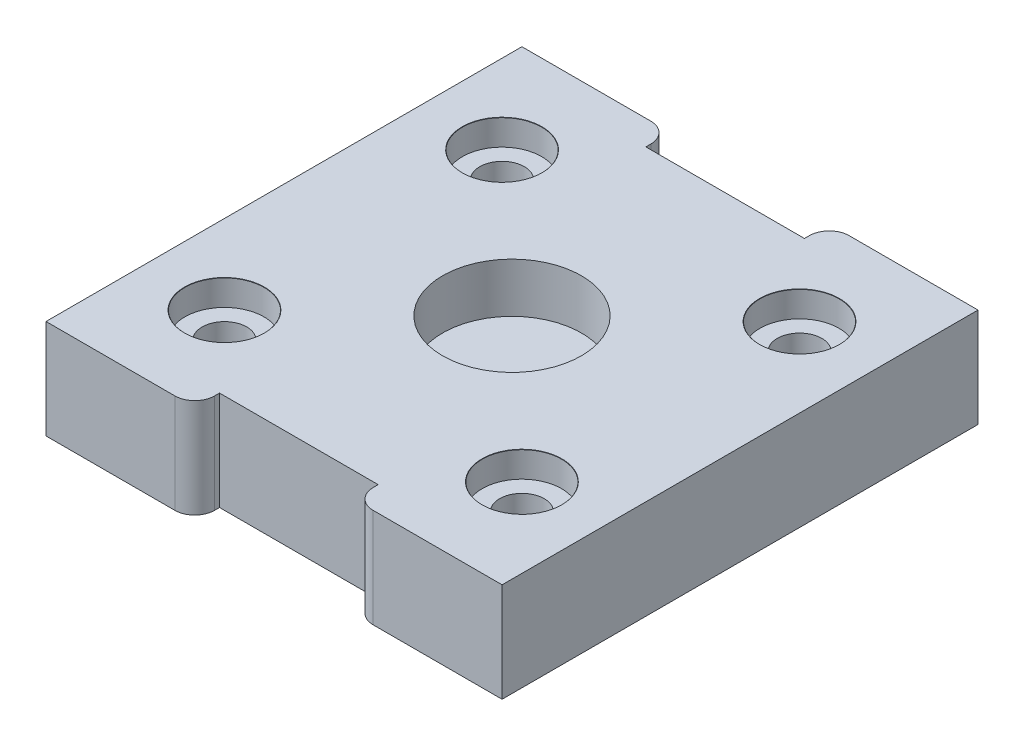
SolidWorks part; units mm, degrees
ref_plane "Front Plane" through (0, 0, 0) normal (0, 0, 1) x (1, 0, 0)
ref_plane "Top Plane" through (0, 0, 0) normal (0, 1, 0) x (1, 0, 0)
ref_plane "Right Plane" through (0, 0, 0) normal (1, 0, 0) x (0, 0, -1)
sketch "Sketch1" plane through (0, 0, 0) normal (0, 0, 1) x (1, 0, 0)
  line L1 (-23, 5) -> (23, 5)
  line L2 (-23, 5) -> (-23, -5)
  line L3 (-23, -5) -> (23, -5)
  line L4 (23, 5) -> (23, -5)
  line L5 (-23, 5) -> (23, -5) construction
  line L6 (-23, -5) -> (23, 5) construction
  point P0 (0, 0)
  dimension "D1" = 46
  dimension "D2" = 10
extrude "Boss-Extrude1" add sketch "Sketch1" along normal blind 48
sketch "Sketch2" plane through (0, 5, 0) normal (0, 1, 0) x (1, 0, 0)
  line L0 (-23, -24) -> (23, -24) construction
  line L1 (-23, -48) -> (-23, 0) construction
  line L2 (23, -48) -> (23, 0) construction
  line L3 (0, -48) -> (0, 0) construction
  line L4 (23, -48) -> (-23, -48) construction
  line L5 (-8, -45.5) -> (8, -45.5)
  line L6 (-8, 2.5) -> (8, 2.5)
  line L7 (-8, 2.5) -> (-8, -2.5)
  line L8 (-8, -2.5) -> (8, -2.5)
  line L9 (8, 2.5) -> (8, -2.5)
  line L10 (-8, 2.5) -> (8, -2.5) construction
  line L11 (-8, -2.5) -> (8, 2.5) construction
  line L12 (8, -50.5) -> (8, -45.5)
  line L13 (-8, -50.5) -> (8, -50.5)
  line L14 (-8, -50.5) -> (-8, -45.5)
  dimension "D1" = 5
  dimension "D2" = 16
extrude "Cut-Extrude1" cut sketch "Sketch2" against normal blind 10
fillet "Fillet1" radius 2 4 edges at (8, 0, 48) (-8, 0, 48) (8, 0, 0) (-8, 0, 0)
hole_wizard "CBORE for M4 Cheese Head Screw1" positions "Sketch3" profile "Sketch4" counterbore size "M4" standard "ISO"
sketch "Sketch3" plane through (0, 5, 0) normal (0, 1, 0) x (1, 0, 0)
  line L0 (0, -45.5) -> (0, -2.5) construction
  line L1 (8, -45.5) -> (-8, -45.5) construction
  line L2 (-8, -2.5) -> (8, -2.5) construction
  line L4 (-23, -24) -> (23, -24) construction
  line L5 (-23, -48) -> (-23, 0) construction
  line L6 (23, -48) -> (23, 0) construction
  line L8 (-15, -10) -> (15, -10) construction
  line L10 (-15, -10) -> (-15, -38) construction
  line L13 (15, -10) -> (15, -38) construction
  line L14 (15, -38) -> (-15, -38) construction
  point P0 (-15, -10)
  point P2 (-15, -38)
  point P4 (15, -38)
  point P6 (15, -10)
  point P44 (0, -24)
  point P45 (-15, -24)
  point P46 (0, -10)
  dimension "D1" = 30
  dimension "D2" = 28
sketch "Sketch4" plane through (-15, 5, 10) normal (1, 0, 0) x (0, 0, 1)
  line L0 (0, 0) -> (0, 11.3519)
  line L1 (0, 11.3519) -> (2.25, 10)
  line L2 (2.25, 10) -> (2.25, 2.6)
  line L3 (2.25, 2.6) -> (4, 2.6)
  line L5 (4, 2.6) -> (4, 0.025)
  line L6 (4, 0.025) -> (4.025, 0)
  line L7 (4.025, 0) -> (0, 0)
  line L8 (-4, 0.025) -> (-4.025, 0) construction
  line L10 (0, 11.3519) -> (-2.25, 10) construction
  line L11 (0, -6.35) -> (0, 107.95) construction
  dimension "Hole Dia." = 4.5
  dimension "Hole Depth" = 10
  dimension "C'Bore Dia." = 8
  dimension "C'Bore Depth" = 2.6
  dimension "Near C'Sink Dia." = 8.05
  dimension "Near C'Sink Angle" = 90
  dimension "Drill Angle" = 118
sketch "Sketch6" plane through (0, 5, 0) normal (0, 1, 0) x (1, 0, 0)
  line L0 (-23, -24) -> (23, -24) construction
  line L1 (-23, -48) -> (-23, 0) construction
  line L2 (23, -48) -> (23, 0) construction
  circle A0 centre (0, -24) radius 7
  dimension "D1" = 14
extrude "Cut-Extrude2" cut sketch "Sketch6" against normal blind 5
